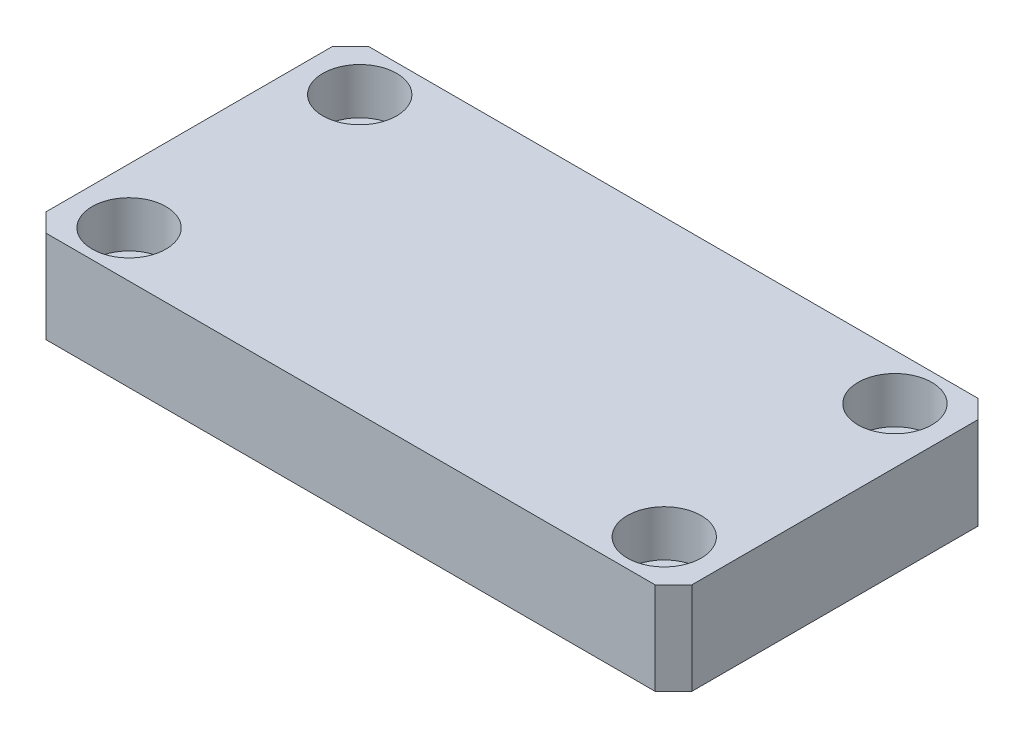
SolidWorks part; units mm, degrees
material "S45C"
ref_plane "前视基准面" through (0, 0, 0) normal (0, 0, 1) x (1, 0, 0)
ref_plane "上视基准面" through (0, 0, 0) normal (0, 1, 0) x (1, 0, 0)
ref_plane "右视基准面" through (0, 0, 0) normal (1, 0, 0) x (0, 0, -1)
sketch "草图1" plane through (0, 0, 0) normal (0, 1, 0) x (1, 0, 0)
  line L1 (-35, -17.5) -> (35, -17.5)
  line L2 (-35, -17.5) -> (-35, 17.5)
  line L3 (-35, 17.5) -> (35, 17.5)
  line L4 (35, -17.5) -> (35, 17.5)
  line L5 (-35, -17.5) -> (35, 17.5) construction
  line L6 (-35, 17.5) -> (35, -17.5) construction
  point P0 (0, 0)
  dimension "D1" = 35
  dimension "D2" = 70
extrude "凸台-拉伸1" add sketch "草图1" along normal mid plane 10
chamfer "倒角1" distance 2 angle 45 4 edges at (-35, 0, -17.5) (35, 0, -17.5) (35, 0, 17.5) (-35, 0, 17.5)
sketch "草图2" plane through (0, 5, 0) normal (0, 1, 0) x (1, 0, 0)
  line L0 (0, 0) -> (40.5341, 0) construction
  line L3 (0, 0) -> (0, 21.6286) construction
  point P0 (-29, 12.5)
  point P2 (-29, -12.5)
  point P4 (29, 12.5)
  point P6 (29, -12.5)
  dimension "D1" = 58
  dimension "D2" = 25
hole_wizard "M4 六角圆柱头螺钉的柱形沉头孔1" positions "草图2" profile "草图3" counterbore size "M4" standard "GB" end condition up to next
sketch "草图3" plane through (-29, 5, -12.5) normal (1, 0, 0) x (0, 0, 1)
  line L0 (0, 0) -> (0, 10)
  line L1 (0, 10) -> (2.25, 10)
  line L3 (2.25, 10) -> (2.25, 5)
  line L4 (2.25, 5) -> (4, 5)
  line L5 (4, 5) -> (4, 0)
  line L7 (4, 0) -> (0, 0)
  line L11 (0, -6.35) -> (0, 107.95) construction
  dimension "通孔孔直径" = 4.5
  dimension "通孔孔深度" = 10
  dimension "柱形沉头孔直径" = 8
  dimension "柱形沉头孔深度" = 5
